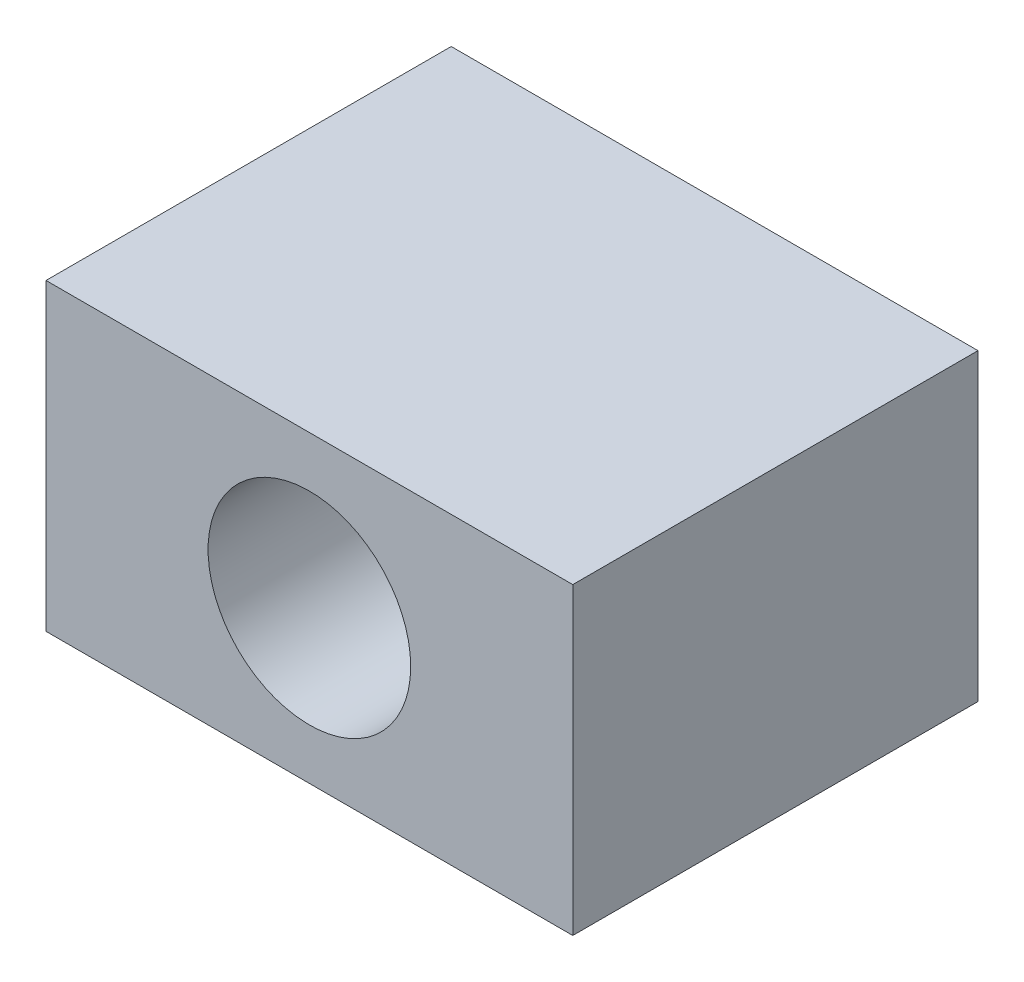
from build123d import *

# Parameters (mm, degrees)
SKETCH1_W           = 26
SKETCH1_H           = 15
SKETCH1_R           = 5
BOSS_EXTRUDE1_DEPTH = 20


with BuildPart() as part:
    # Sketch1 → Boss-Extrude1 (new body)
    with BuildSketch(Plane.XY):
        Rectangle(SKETCH1_W, SKETCH1_H)
        Circle(SKETCH1_R, mode=Mode.SUBTRACT)
    extrude(amount=BOSS_EXTRUDE1_DEPTH)


solid = part.part
